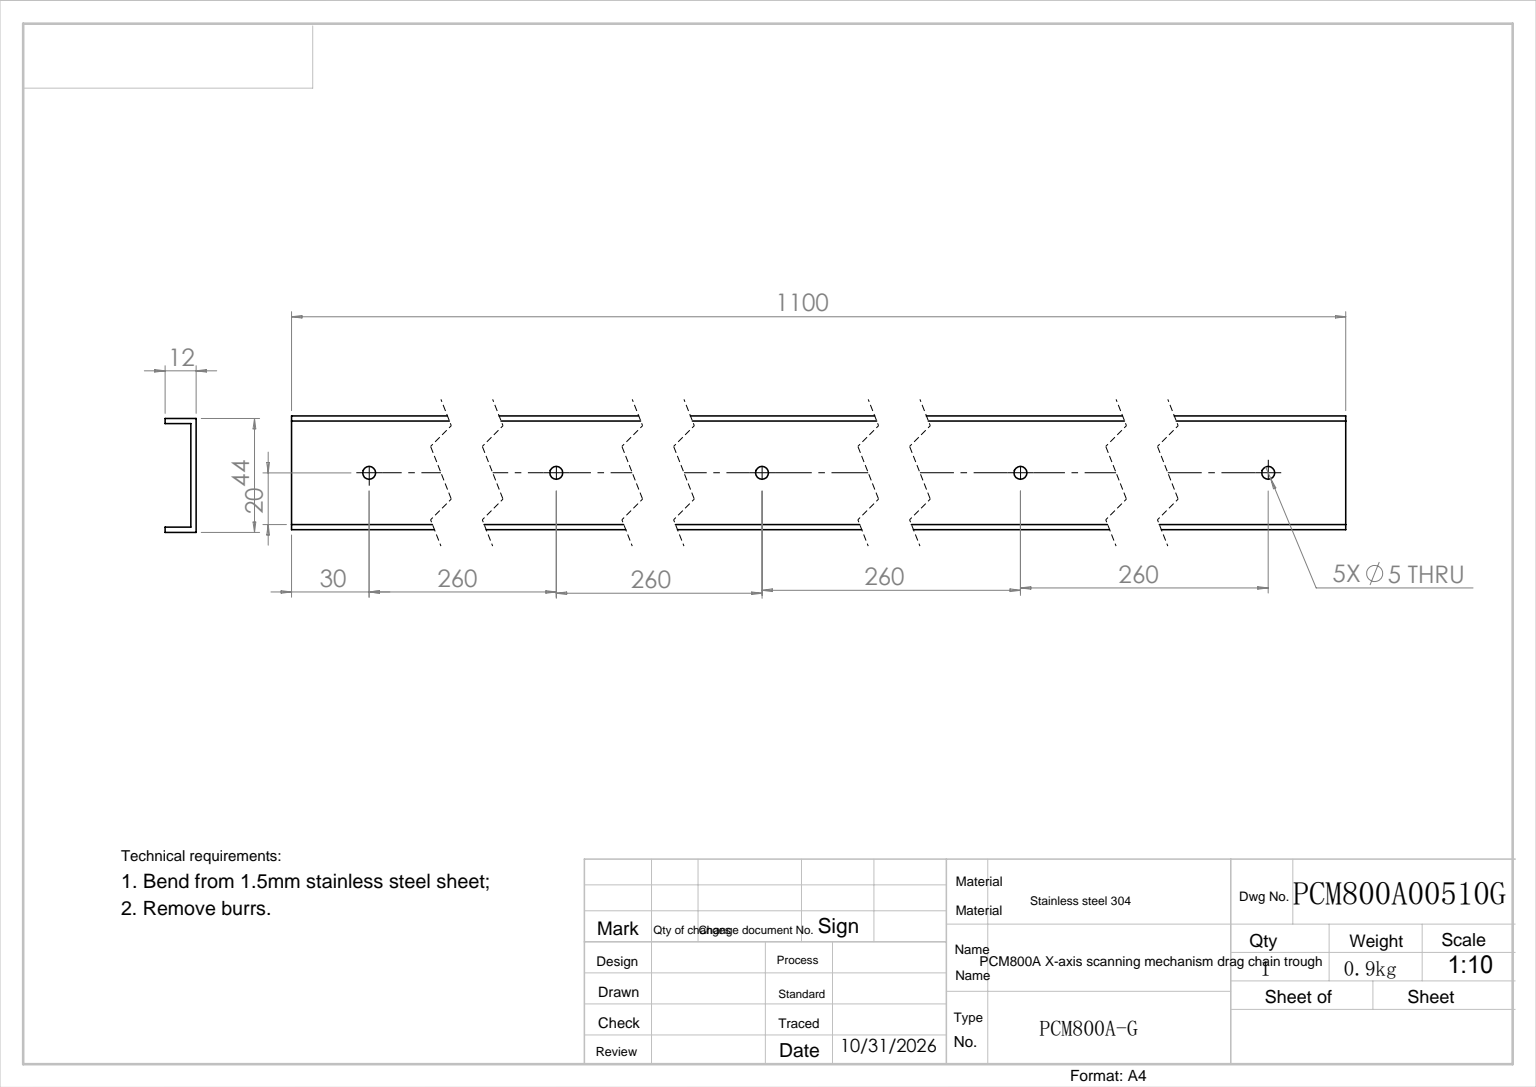
from build123d import *

# Parameters (mm, degrees)
EXTRUDE_1_DEPTH        = 1100
SKETCH_2_R             = 2.5
CUT_EXTRUDE_1_DEPTH    = 1101.846946673
PATTERN_LINEAR_1_COUNT = 5
PATTERN_LINEAR_1_PITCH = 260


with BuildPart() as part:
    # 草图1 → 凸台-拉伸1 (new body)
    with BuildSketch(Plane.XY):
        Polygon((0, 0), (0, -10), (40, -10), (40, 0), (42, 0), (42, -12), (-2, -12), (-2, 0), align=None)
    extrude(amount=EXTRUDE_1_DEPTH)

    # 草图2 → 切除-拉伸1 (cut, through all)
    with BuildSketch(Plane(origin=(0, -10, 0), x_dir=(1, 0, 0), z_dir=(0, 1, 0))):
        with Locations(Location((20, -30, 0), (0, 0, 270))):
            Circle(SKETCH_2_R)
    cut_extrude_1 = extrude(amount=-CUT_EXTRUDE_1_DEPTH, mode=Mode.SUBTRACT)

    # 阵列(线性)1: 切除-拉伸1 ×5
    with Locations(*[(0, 0, i * PATTERN_LINEAR_1_PITCH) for i in range(1, PATTERN_LINEAR_1_COUNT)]):
        add(cut_extrude_1, mode=Mode.SUBTRACT)


solid = part.part
